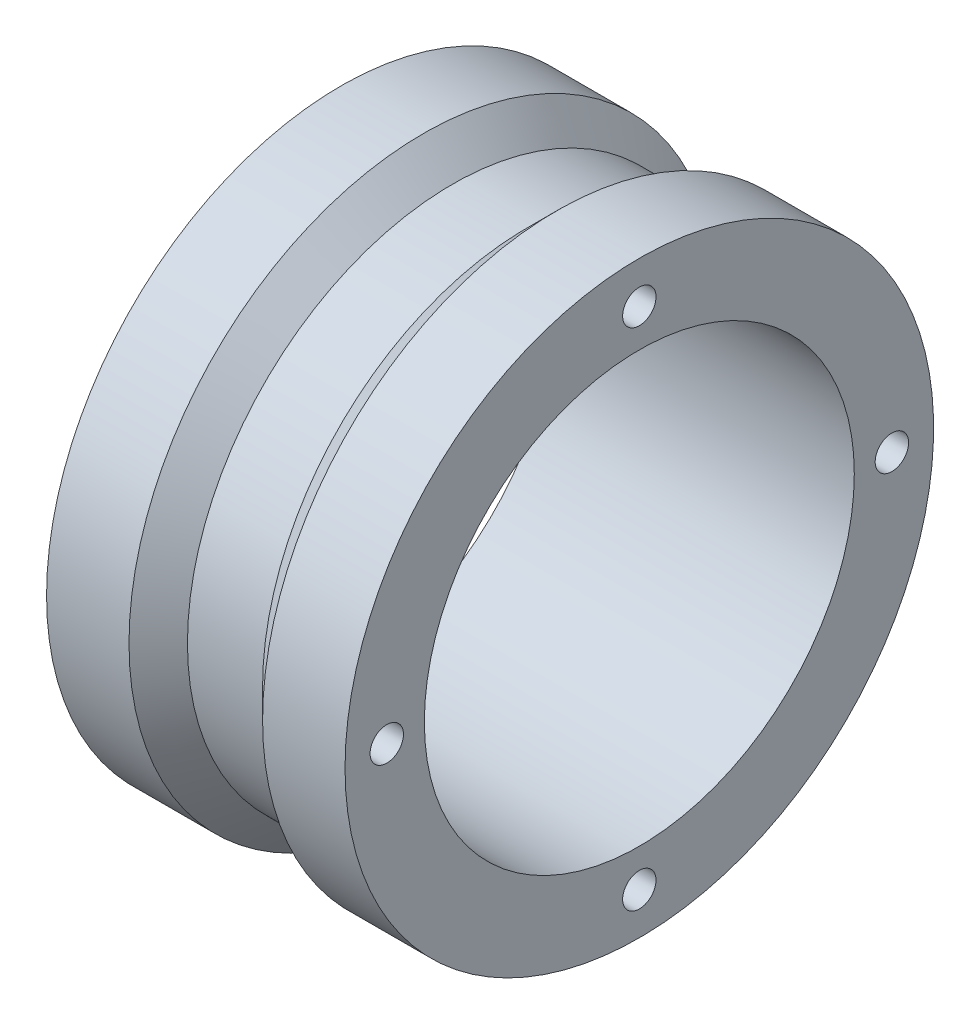
from build123d import *

# Parameters (mm, degrees)
SKETCH4_R          = 4
CUT_EXTRUDE1_DEPTH = 13
CUT_EXTRUDE2_START = -13
SKETCH5_R          = 4
CUT_EXTRUDE2_DEPTH = 13


with BuildPart() as part:
    # Sketch2 → Revolve1 (revolve)
    with BuildSketch(Plane.XY, mode=Mode.PRIVATE) as revolve1_sk:
        Polygon((-37.225396825, 70.5), (-37.225396825, 51.5), (34.274603175, 51.5), (34.274603175, 70.5), (14.524603175, 70.5), (7.524603175, 63.5), (-10.475396825, 63.5), (-17.475396825, 70.5), align=None)
    revolve(revolve1_sk.sketch.rotate(Axis((-86.707936508, 0, 0), (1, 0, 0)), 90), axis=Axis((-86.707936508, 0, 0), (1, 0, 0)))

    # Sketch4 → Cut-Extrude1 (cut)
    with BuildSketch(Plane.ZY.offset(37.225396825)):
        with Locations((0, -60.5)):
            Circle(SKETCH4_R)
        with Locations((-60.5, 0)):
            Circle(SKETCH4_R)
        with Locations((0, 60.5)):
            Circle(SKETCH4_R)
        with Locations((60.5, 0)):
            Circle(SKETCH4_R)
    extrude(amount=-CUT_EXTRUDE1_DEPTH, mode=Mode.SUBTRACT)

    # Sketch5 → Cut-Extrude2 (cut)
    with BuildSketch(Plane(origin=(34.274603175, 0, 0), x_dir=(0, 0, -1), z_dir=(1, 0, 0)).offset(CUT_EXTRUDE2_START)):
        with Locations(Location((0, -60.5, 0), (0, 0, 180))):
            Circle(SKETCH5_R)
        with Locations(Location((-60.5, 0, 0), (0, 0, 180))):
            Circle(SKETCH5_R)
        with Locations(Location((0, 60.5, 0), (0, 0, 180))):
            Circle(SKETCH5_R)
        with Locations(Location((60.5, 0, 0), (0, 0, 180))):
            Circle(SKETCH5_R)
    extrude(amount=CUT_EXTRUDE2_DEPTH, mode=Mode.SUBTRACT)


solid = part.part
